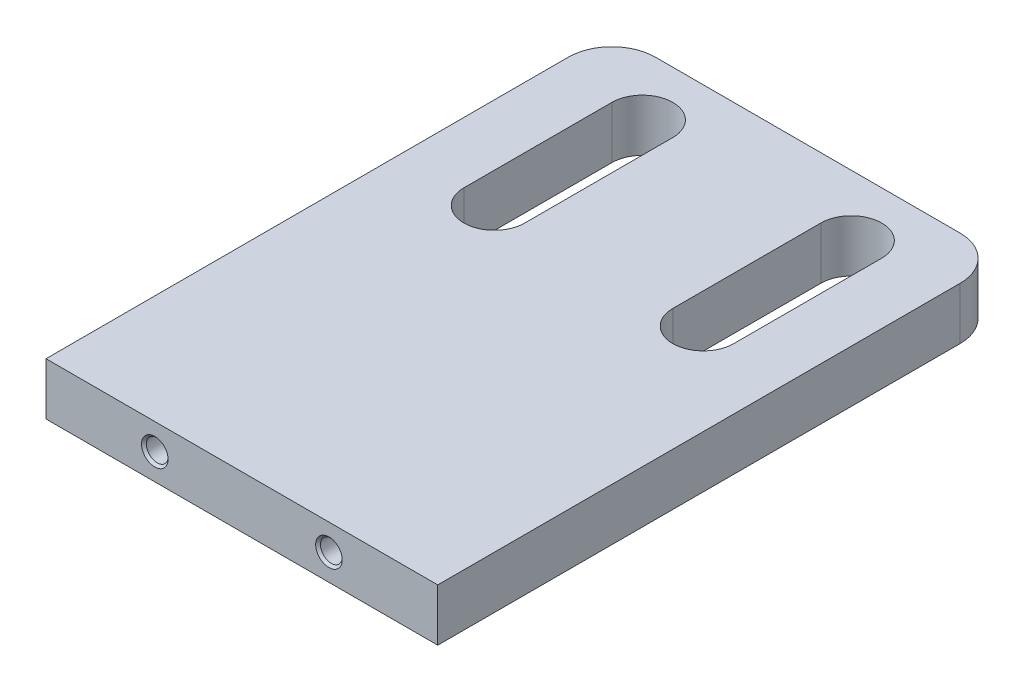
from build123d import *

# Parameters (mm, degrees)
SKETCH1_W                   = 45
SKETCH1_H                   = 65
BOSS_EXTRUDE1_DEPTH         = 6
CUT_EXTRUDE1_DEPTH          = 6
FILLET2_R                   = 5
M3_TAPPED_HOLE1_D           = 2.5
M3_TAPPED_HOLE1_DEPTH       = 13.5
M3_TAPPED_HOLE1_CSINK_D     = 3.05
M3_TAPPED_HOLE1_CSINK_ANGLE = 90
M3_TAPPED_HOLE1_TIP         = 0.751075774


with BuildPart() as part:
    # Sketch1 → Boss-Extrude1 (new body)
    with BuildSketch(Plane(origin=(0, 0, 0), x_dir=(1, 0, 0), z_dir=(0, 1, 0))):
        Rectangle(SKETCH1_W, SKETCH1_H)
    extrude(amount=BOSS_EXTRUDE1_DEPTH)

    # Sketch6 → Cut-Extrude1 (cut)
    with BuildSketch(Plane(origin=(0, 6, 0), x_dir=(1, 0, 0), z_dir=(0, 1, 0))):
        with BuildLine():
            Line((-8.5, 25.5), (-8.5, 8.5))
            ThreePointArc((-8.5, 8.5), (-12, 5), (-15.5, 8.5))
            Line((-15.5, 8.5), (-15.5, 25.5))
            ThreePointArc((-15.5, 25.5), (-12, 29), (-8.5, 25.5))
        make_face()
        with BuildLine():
            Line((8.5, 25.5), (8.5, 8.5))
            ThreePointArc((8.5, 8.5), (12, 5), (15.5, 8.5))
            Line((15.5, 8.5), (15.5, 25.5))
            ThreePointArc((15.5, 25.5), (12, 29), (8.5, 25.5))
        make_face()
    extrude(amount=-CUT_EXTRUDE1_DEPTH, mode=Mode.SUBTRACT)

    # Fillet2
    fillet2_edges = [part.edges().sort_by_distance(p)[0] for p in [
        (-22.5, 3, -32.5),
        (22.5, 3, -32.5),
    ]]
    fillet(fillet2_edges, radius=FILLET2_R)

    # M3 Tapped Hole1
    with Locations(Plane.XY.offset(32.5)):
        with Locations((-10, 3), (10, 3)):
            CounterSinkHole(M3_TAPPED_HOLE1_D / 2, M3_TAPPED_HOLE1_CSINK_D / 2, depth=M3_TAPPED_HOLE1_DEPTH, counter_sink_angle=M3_TAPPED_HOLE1_CSINK_ANGLE)
            with Locations((0, 0, -(M3_TAPPED_HOLE1_DEPTH + M3_TAPPED_HOLE1_TIP / 2))):  # 118° drill point
                Cone(0, M3_TAPPED_HOLE1_D / 2, M3_TAPPED_HOLE1_TIP, mode=Mode.SUBTRACT)


solid = part.part
